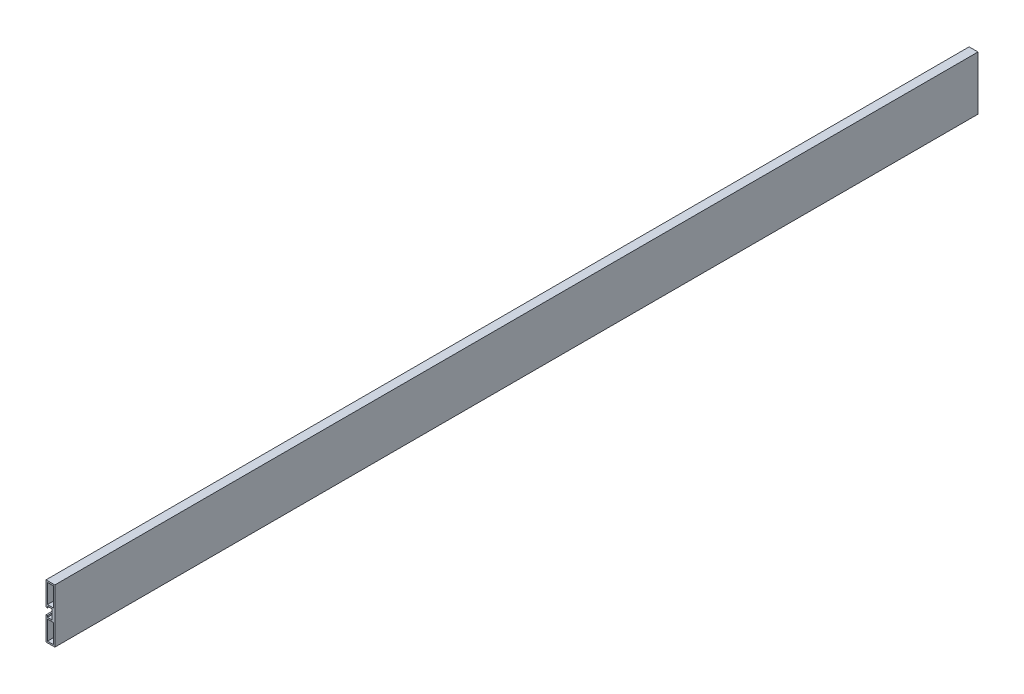
from build123d import *

# Parameters (mm, degrees)
SKETCH_1_W      = 8
SKETCH_1_H      = 26
EXTRUDE_1_DEPTH = 625


with BuildPart() as part:
    # 草图1 → 凸台-拉伸1 (new, symmetric)
    with BuildSketch(Plane.XY):
        Polygon((-12, 4.5), (-10, 4.5), (-10, 6.5), (-4, 6.5), (-4, -6.5), (-10, -6.5), (-10, -4.5), (-12, -4.5), (-12, -36.5), (0, -36.5), (0, 36.5), (-12, 36.5), align=None)
        with Locations((-6, -21.5)):
            Rectangle(SKETCH_1_W, SKETCH_1_H, mode=Mode.SUBTRACT)
        with Locations((-6, 21.5)):
            Rectangle(SKETCH_1_W, SKETCH_1_H, mode=Mode.SUBTRACT)
    extrude(amount=EXTRUDE_1_DEPTH, both=True)


solid = part.part
